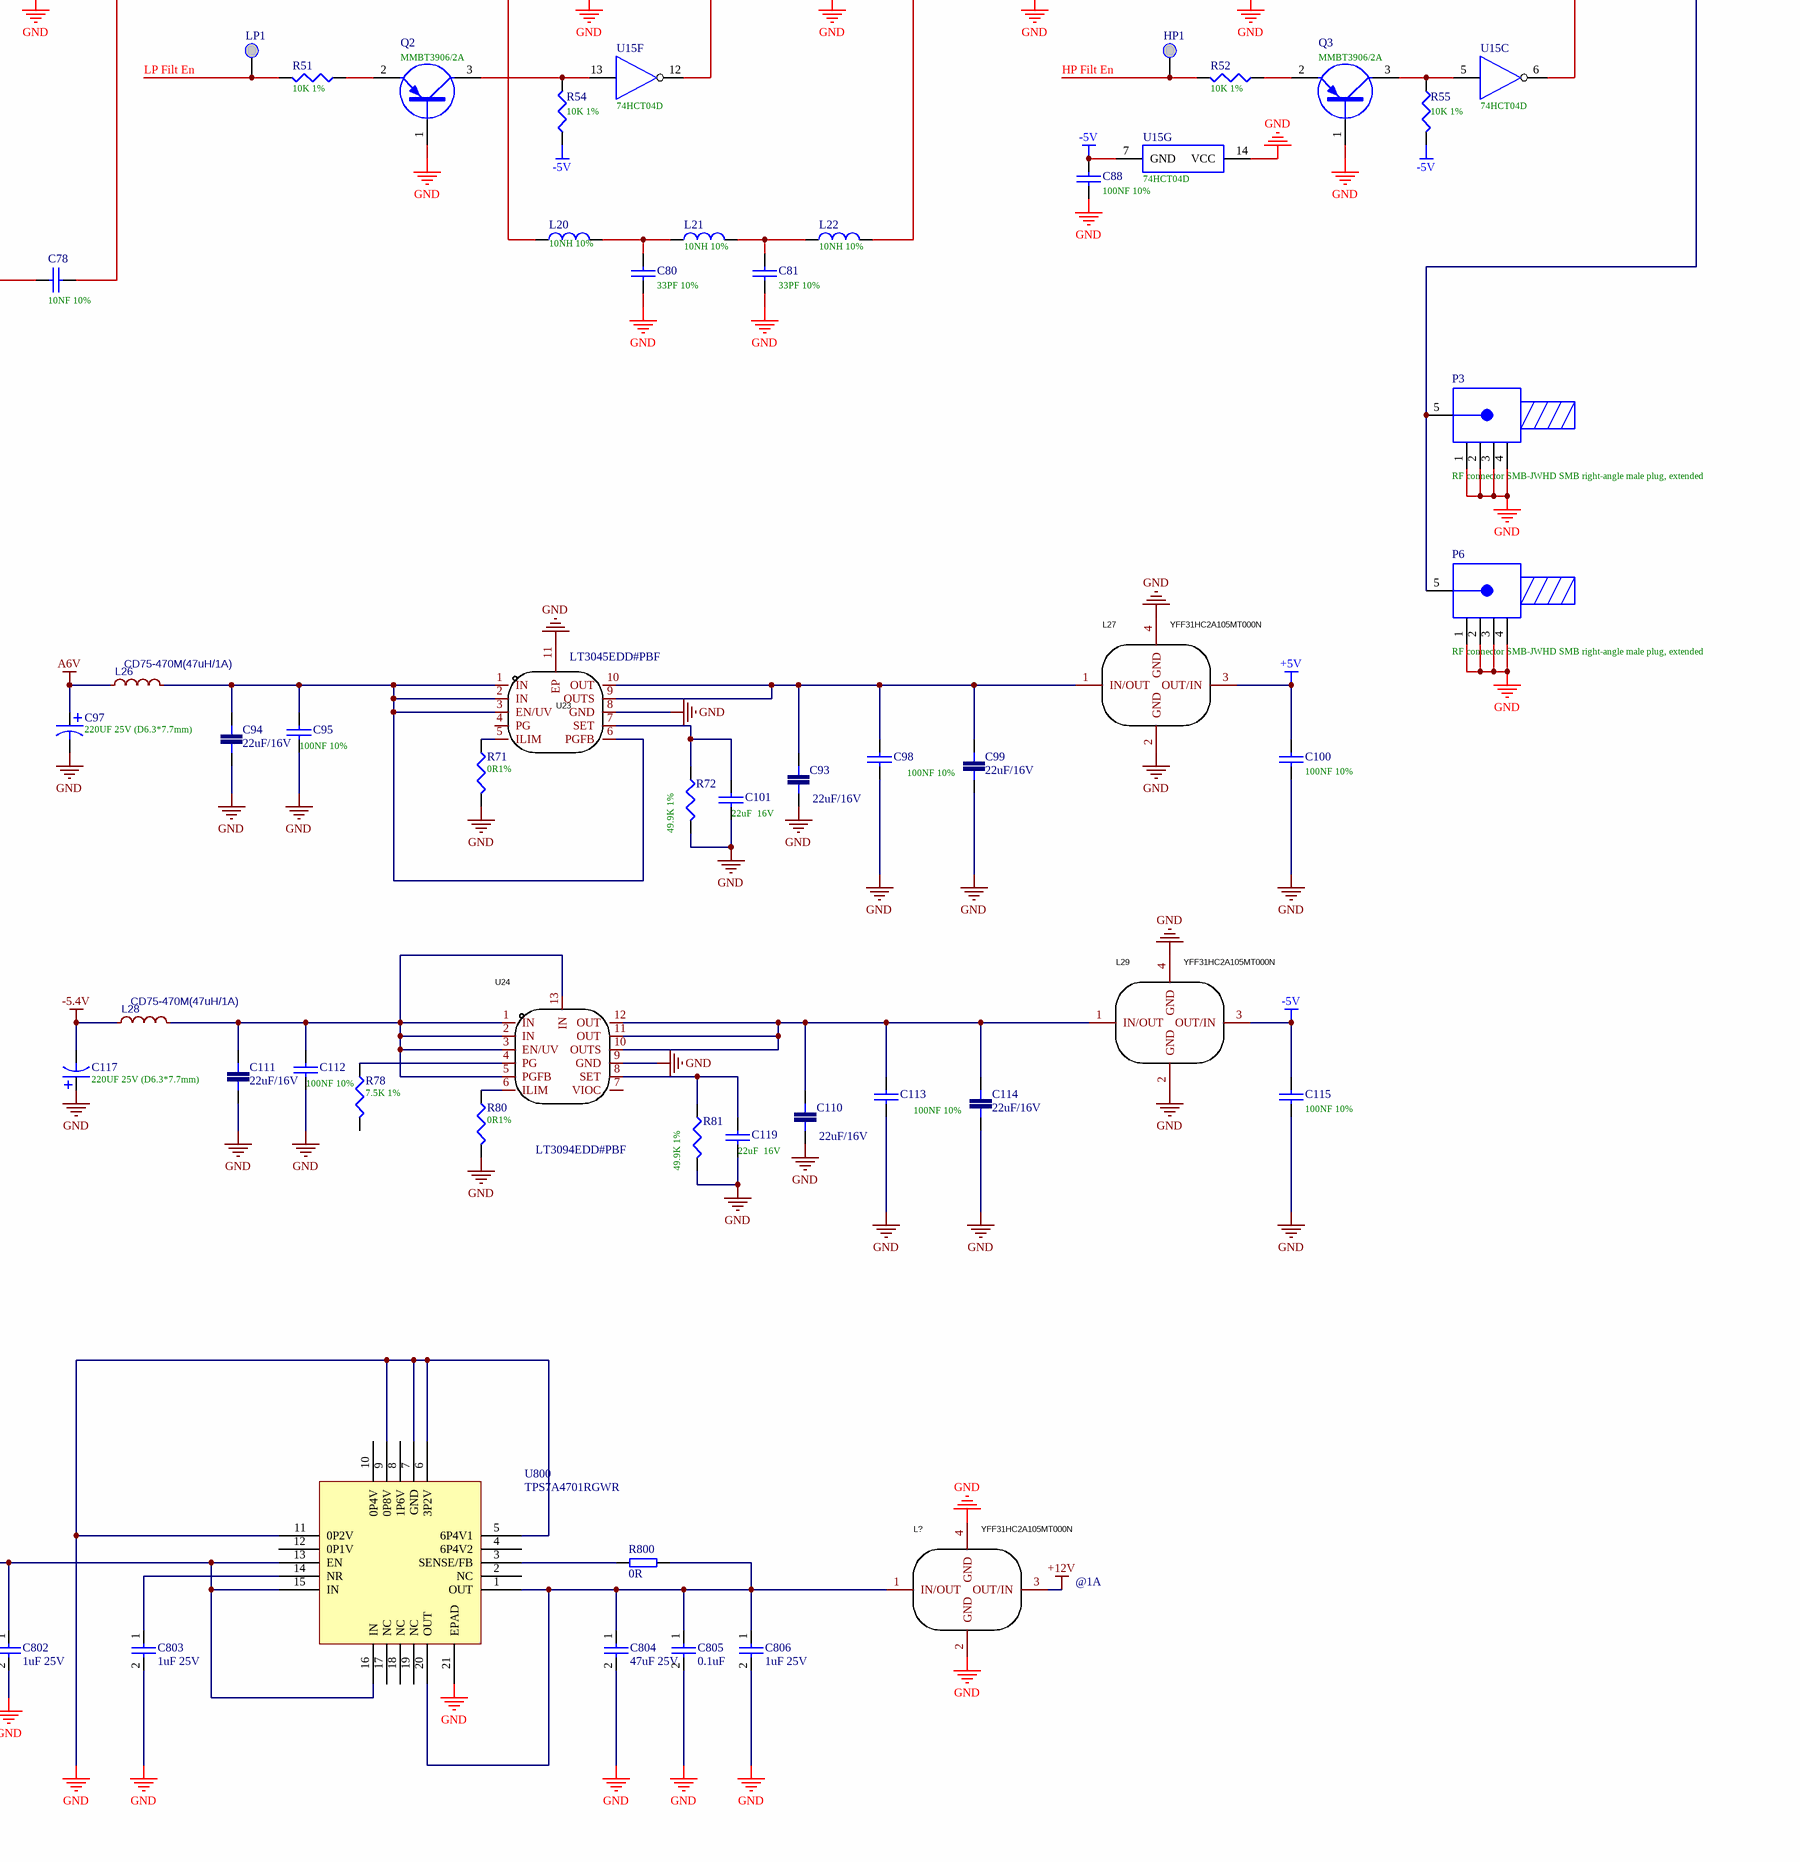
[diagram p0: PCBE109560.SchDoc, bottom right]
# Altium schematic sheet PCBE109560.SchDoc (part 2 of 2)

## Parts
1  (no value)  [DIP-1]
+1  (no value)  [DIP-1]
+2  (no value)  [DIP-1]
C4  20PF 10%  [0805C]
C5  330PF 10%  [1812C]
C6  22PF 10%  [1812C-2]
C7  22uF/16V  [0805]
C8  22uF/16V  [0805]
C9  100NF 10%  [0603]
C10  220UF 25V (D6.3*7.7mm)  [CAP-SMD_BD6.3-L6.6-W6.6-FD]
C11  100NF 10%  [0603]
C12  22uF/16V  [0805]
C13  100NF 10%  [0805R]
C14  22uF  16V  [0805]
C15  100NF 10%  [0805R]
C16  47PF 10%  [1812C-2]
C17  100PF 10%  [1812C-2]
C18  20PF 10%  [0805R]
C20  100NF 10%  [0805R]
C21  100NF 10%  [0805R]
C31  100NF 10%  [0805R]
C32  100NF 10%  [0805R]
C34  100NF 10%  [0805R]
C35  100NF 10%  [0805R]
C36  100NF 10%  [0805R]
C37  100NF 10%  [0805R]
C39  100NF 10%  [0805R]
C40  100NF 10%  [0805R]
C41  100NF 10%  [0805R]
C42  100NF 10%  [0805R]
C43  100NF 10%  [0805R]
C44  100NF 10%  [0805R]
C45  100NF 10%  [0805R]
C46  100NF 10%  [0805R]
C47  100NF 10%  [0805R]
C48  100NF 10%  [0805R]
C49  22uF 25V  [CAP-SMD_L6.0-W3.2-R-RD]
C50  100NF 10%  [0805R]
C51  100NF 10%  [0805R]
C52  100NF 10%  [0805R]
C53  3.3NF 10%  [0805R]
C54  100NF 10%  [0805R]
C55  330PF 10%  [0805R]
C56  330PF 10%  [0805R]
C57  100NF 10%  [0805R]
C58  33PF 10%  [0805R]
C59  33PF 10%  [0805R]
C60  100NF 10%  [0805R]
C61  100NF 10%  [0805R]
C62  100NF 10%  [0805R]
C63  100NF 10%  [0805R]
C64  100NF 10%  [0805R]
C65  33PF 10%  [0805R]
C66  33PF 10%  [0805R]
C67  100NF 10%  [0805R]
C68  39PF 10%  [0805R]
C69  100NF 10%  [0805R]
C70  25V 1UF Type A  [0805C-2]
C71  25V 1UF Type A  [0805C-2]
C72  100NF 10%  [0805R]
C73  25V 1UF Type A  [0805C-2]
C74  100NF 10%  [0805R]
C75  100NF 10%  [0805R]
C76  10NF 10%  [0805R]
C77  10NF 10%  [0805R]
C78  10NF 10%  [0805R]
C79  100NF 10%  [0603C]
C80  33PF 10%  [0805R]
C81  33PF 10%  [0805R]
C82  100NF 10%  [0805R]
C83  100NF 10%  [0805R]
C84  100NF 10%  [0805R]
C85  100NF 10%  [0805R]
C86  25V 1UF Type A  [0805C-2]
C87  3pF( ±0.1pF)  [0805R]
C88  100NF 10%  [0805R]
C89  100NF 10%  [0805R]
C90  100NF 10%  [0805R]
C93  22uF/16V  [0805]
C94  22uF/16V  [0805]
C95  100NF 10%  [0603]
C96  100NF 10%  [0805R]
C97  220UF 25V (D6.3*7.7mm)  [CAP-SMD_BD6.3-L6.6-W6.6-FD]
C98  100NF 10%  [0603]
C99  22uF/16V  [0805]
C100  100NF 10%  [0805R]
C101  22uF  16V  [0805]
C102  100NF 10%  [0805R]
C103  100NF 10%  [0805R]
C104  100NF 10%  [0805R]
C105  100NF 10%  [0805R]
C106  100NF 10%  [0805R]
C107  100NF 10%  [0805R]
C109  100NF 10%  [0805R]
C110  22uF/16V  [0805]
C111  22uF/16V  [0805]
C112  100NF 10%  [0603]
C113  100NF 10%  [0603]
C114  22uF/16V  [0805]
C115  100NF 10%  [0805R]
C116  100NF 10%  [0805R]
C117  220UF 25V (D6.3*7.7mm)  [CAP-SMD_BD6.3-L6.6-W6.6-FD]
C118  100NF 10%  [0805R]
C119  22uF  16V  [0805]
C122  100NF 10%  [0805R]
C123  100NF 10%  [0805R]
C124  100NF 10%  [0805R]
C125  100NF 10%  [0805R]
C128  100NF 10%  [0805R]
C129  100NF 10%  [0805R]
C130  100NF 10%  [0805R]
C800  47uF 25V  [1206]
C801  0.1uF  [0402]
C802  1uF 25V  [0402]
C803  1uF 25V  [0402]
C804  47uF 25V  [1206]
C805  0.1uF  [0402]
C806  1uF 25V  [0402]
Clk1  (no value)  [DIP-1]
D1  BAV99/A7  [SOT-23]
D2  GF1M-E3/67A/GM  [1808D]
D3  GF1M-E3/67A/GM  [1808D]
D4  GF1M-E3/67A/GM  [1808D]
D5  GF1M-E3/67A/GM  [1808D]
D8  BAV99/A7  [SOT-23-2]
D9  BAV99/A7  [SOT-23-2]
D10  BAV99/A7  [SOT-23-2]
D11  BAV99/A7  [SOT-23-2]
D12  BAV99/A7  [SOT-23-2]
Data1  (no value)  [DIP-1]
HP1  (no value)  [DIP-1]
J1  RF connector  [DIP-J-2]
J2  RF connector  [DIP-J-2]
L2  15UH 5%  [1005R]
L3  BLM21PG221SN1D(220Ω@100MHz)  [0805R]
L4  YFF31HC2A105MT000N  [FILTER-SMD_4P-L3.2-W1.6-L_YFF31HC]
L5  6.8UH 10%  [0805R]
L8  YFF31HC2A105MT000N  [FILTER-SMD_4P-L3.2-W1.6-L_YFF31HC]
L9  BLM21PG221SN1D(220Ω@100MHz  [0805R]
L10  10NH 10%  [0805R]
L11  10NH 10%  [0805R]
L12  10NH 10%  [0805R]
L13  YFF31HC2A105MT000N  [FILTER-SMD_4P-L3.2-W1.6-L_YFF31HC]
L14  BLM21PG221SN1D(220Ω@100MHz  [0805R]
L15  4.7UH 5%  [1005L]
L16  1UH 5%  [0805R]
L17  BLM21PG221SN1D(220Ω@100MHz)  [0805R]
L18  BLM21PG221SN1D(220Ω@100MHz  [0805R]
L19  BLM21PG221SN1D(220Ω@100MHz  [0805R]
L20  10NH 10%  [0805R]
L21  10NH 10%  [0805R]
L22  10NH 10%  [0805R]
L23  YFF31HC2A105MT000N  [FILTER-SMD_4P-L3.2-W1.6-L_YFF31HC]
L24  YFF31HC2A105MT000N  [FILTER-SMD_4P-L3.2-W1.6-L_YFF31HC]
L25  BLM21PG221SN1D(220Ω@100MHz  [0805R]
L26  CD75-470M(47uH/1A)  [IND-SMD_L7.8-W7.0-A]
L27  YFF31HC2A105MT000N  [FILTER-SMD_4P-L3.2-W1.6-L_YFF31HC]
L28  CD75-470M(47uH/1A)  [IND-SMD_L7.8-W7.0-A]
L29  YFF31HC2A105MT000N  [FILTER-SMD_4P-L3.2-W1.6-L_YFF31HC]
L31  BLM21PG221SN1D(220Ω@100MHz  [0805R]
L32  BLM21PG221SN1D(220Ω@100MHz  [0805R]
L808  NFM15PC104R1A3D  [FILTER-SMD_0402-3P-L1.0-W0.5-T]
L809  NFM15PC104R1A3D  [FILTER-SMD_0402-3P-L1.0-W0.5-T]
L810  NFM15PC104R1A3D  [FILTER-SMD_0402-3P-L1.0-W0.5-T]
L811  NFM15PC104R1A3D  [FILTER-SMD_0402-3P-L1.0-W0.5-T]
L812  NFM15PC104R1A3D  [FILTER-SMD_0402-3P-L1.0-W0.5-T]
L813  NFM15PC104R1A3D  [FILTER-SMD_0402-3P-L1.0-W0.5-T]
L?  YFF31HC2A105MT000N  [FILTER-SMD_4P-L3.2-W1.6-L_YFF31HC]
LP1  (no value)  [DIP-1]
P1  Header 20X2  [N0.8mm/40Pin-Plug]
P2  Header 4X2  [N0.8mm/8Pin-SOCKET]
P3  RF connector SMB-JWHD SMB right-angle male plug, extended  [DIP-P-2]
P4  Header 20X2  [N0.8mm/40Pin-Plug]
P5  Header 20X2  [N0.8mm/40Pin-Plug]
P6  RF connector SMB-JWHD SMB right-angle male plug, extended  [DIP-P-2]
Q1  MJD31C  [SOT-252-2]
Q2  MMBT3906/2A  [SOT-23]
Q3  MMBT3906/2A  [SOT-23]
Q4  MMBT3906/2A  [SOT-23]
R6  2K 5%  [0603R]
R7  NC  [AXIAL-0.51]
R8  3.9K 5% 1/2W  [AXIAL-0.51]
R9  3.9K 5% 1/2W  [AXIAL-0.51]
R10  3.9K 5% 1/2W  [AXIAL-0.51]
R11  3.9K 5% 1/2W  [AXIAL-0.51]
R13  0R1%  [0603]
R14  49.9K 1%  [0603]
R15  4.99K 1%  [0805R]
R16  2K 1%  [0805R]
R17  49.9R 1% 1/4W  [AXIAL-0.4]
R20  100R 1% 1/4W  [AXIAL-0.4]
R23  100R 1% 1/4W  [AXIAL-0.4]
R27  4.87K 1%  [0805R]
R28  4.87K 1%  [0805R]
R29  4.87K 1%  [0805R]
R30  4.87K 1%  [0805R]
R31  4.87K 1%  [0805R]
R32  10K 1%  [0805R]
R33  100K 1%  [0805R]
R34  100K 1%  [0805R]
R35  49.9R 1%  [0805R]
R36  49.9R 1%  [0805R]
R37  49.9R 1%  [0805R]
R38  49.9R 1%  [0805R]
R39  49.9R 1%  [0805R]
R40  49.9R 1% 1/4W  [R-SMD_L3.5-W1.5]
R41  10K 1%  [0805R]
R42  4.87K 1%  [0805R]
R43  4.87K 1%  [0805R]
R44  4.87K 1%  [0805R]
R45  4.87K 1%  [0805R]
R46  169R 1%  [0805R]
R47  169R 1%  [0805R]
R48  169R 1%  [0805R]
R49  49.9R 1%  [0805R]
R50  49.9R 1%  [0805R]
R51  10K 1%  [0805R]
R52  10K 1%  [0805R]
R53  10K 1%  [0805R]
R54  10K 1%  [0805R]
R55  10K 1%  [0805R]
R56  10K 1%  [0805R]
R57  10K 1%  [0805R]
R58  49.9R 1%  [0805R]
R59  4.99K 1%  [0805R]
R60  49.9R 1%  [R-SMD_L3.5-W1.5]
R61  30R 1%  [R-SMD_L3.5-W1.5]
R62  169R 1%  [0805R]
R63  169R 1%  [0805R]
R64  169R 1%  [0805R]
R65  49.9R 1%  [0805R]
R66  49.9R 1%  [0805R]
R67  49.9R 1%  [0805R]
R68  49.9R 1%  [0805R]
R69  120R 1%  [R-SMD_L3.5-W1.5]
R70  169R 1%  [0805R]
R71  0R1%  [0603]
R72  49.9K 1%  [0603]
R73  169R 1%  [0805R]
R74  NC  [0805R]
R75  169R 1%  [0805R]
R77  169R 1%  [0805R]
R78  7.5K 1%  [0603]
R80  0R1%  [0603]
R81  49.9K 1%  [0603]
R82  100K 1%  [0805R]
R83  10K 1%  [0805R]
R84  169R 1%  [0805R]
R800  0R  [0402]
RE1  AGQ210A4HZ  [RELAY-SMD_PANASONIC_AGQ2X0AXX]
RE2  AGQ210A4HZ  [RELAY-SMD_PANASONIC_AGQ2X0AXX]
RE3  AGQ210A4HZ  [RELAY-SMD_PANASONIC_AGQ2X0AXX]
RE4  AGQ210A4HZ  [RELAY-SMD_PANASONIC_AGQ2X0AXX]
RE5  AGQ210A4HZ  [RELAY-SMD_PANASONIC_AGQ2X0AXX]
Strobe1  (no value)  [DIP-1]
U4  LT3045EDD#PBF  [DFN-10_L3.0-W3.0-P0.50-BL-EP]
U6  74HCT123D  [SOIC-16_L9.9-W3.9-P1.27-LS6.0-BL]
U8  MAX504CSD+T  [SO-14]
U9  SW-239  [SO-8]
U11  SW-239  [SO-8]
U12  SW-239  [SO-8]
U13  SW-239  [SO-8]
U14  SW-239  [SO-8]
U15  74HCT04D  [SO-14]  (parts A,B,C,D,E,F,G of 7)
U16  AT-250(MAAV-007941)  [SO-8]
U17  MAR-3SM/A03  [LCC4]
U18  MAR-6SM/A06  [LCC4]
U19  MAR-6SM/A06  [LCC4]
U20  MAR-3SM/A03  [LCC4]
U21  MAX4106ESA+T  [SO-8]
U22  MIC4420CM  [SO-8]
U23  LT3045EDD#PBF  [DFN-10_L3.0-W3.0-P0.50-BL-EP]
U24  LT3094EDD#PBF  [WDFN-12_L3.0-W3.0-P0.45-BL-EP]
U25  AT65-0263  [SO-16]
U100  SW-239  [SO-8]
U800  TPS7A4701RGWR  [QFN-20]

## Nets
+5V: C100.1 L27.3(OUT/IN) L808.3(OUTPUT) L811.3(OUTPUT) L812.3(OUTPUT) U8.3(~{CLR})
+12.5V: +2.1 C106.1 C800.1 C801.1 C802.1 P5.31 P5.32 P5.33 P5.34 P5.35 P5.36 P5.37 P5.38 P5.39 P5.40 U800.13(EN) U800.15(IN) U800.16(IN)
+12V: C122.1 C123.1 C124.2 C125.2 L8.1(IN/OUT) L13.1(IN/OUT) L?.3(OUT/IN) U22.1(VS) U22.8(VS)
-5.4V: +1.1 C107.1 C117.2 L28.2 P5.1 P5.2 P5.3 P5.4 P5.5 P5.6 P5.7 P5.8 P5.9 P5.10
-5V: C88.2 C115.2 L29.3(OUT/IN) L809.1(INPUT) L810.3(OUTPUT) L813.3(OUTPUT) R54.1 R55.2 R57.1 U15.7(GND)
A6V: 1.1 C10.1 C97.1 C103.2 L3.1 L26.2 P5.17 P5.18 P5.19 P5.20 P5.21 P5.22 P5.23 P5.24
GND: C5.1 C6.2 C7.1 C8.1 C9.2 C10.2 C11.2 C12.1 C13.2 C14.2 C15.1 C18.2 C20.1 C21.1 C31.1 C32.1 C34.1 C35.1 C36.2 C37.2 C39.2 C40.2 C42.2 C43.1 C44.2 C45.2 C46.2 C47.1 C48.1 C49.2 C50.2 C57.2 C60.2 C61.1 C62.1 C63.1 C64.1 C65.2 C66.1 C70.1 C71.1 C72.2 C73.1 C74.1 C75.1 C80.1 C81.1 C83.2 C84.2 C85.1 C86.2 C88.1 C89.2 C90.2 C93.1 C94.1 C95.2 C96.2 C97.2 C98.2 C99.1 C100.2 C101.2 C102.2 C103.1 C104.2 C105.1 C106.2 C107.2 C109.2 C110.1 C111.1 C112.2 C113.2 C114.1 C115.1 C117.1 C118.2 C119.2 C122.2 C123.2 C124.1 C125.1 C128.1 C129.1 C130.2 C800.2 C801.2 C802.2 C803.2 C804.2 C805.2 C806.2 D1.3 D2.2(K) D11.2 D12.1 J1.1 J1.2 J1.3 J1.4 J2.1 J2.2 J2.3 J2.4 L2.2 L4.2(GND) L4.4(GND) L8.2(GND) L8.4(GND) L13.2(GND) L13.4(GND) L15.2 L16.1 L23.2(GND) L23.4(GND) L24.2(GND) L24.4(GND) L27.2(GND) L27.4(GND) L29.2(GND) L29.4(GND) L808.2(GND) L809.2(GND) L810.2(GND) L811.2(GND) L812.2(GND) L813.2(GND) L?.2(GND) L?.4(GND) P1.5 P1.6 P1.11 P1.12 P1.17 P1.18 P1.20 P1.23 P1.24 P1.29 P1.30 P1.35 P1.36 P2.1 P2.3 P2.5 P2.7 P3.1 P3.2 P3.3 P3.4 P4.5 P4.6 P4.11 P4.12 P4.17 P4.18 P4.23 P4.24 P4.29 P4.30 P4.35 P4.36 P5.11 P5.12 P5.13 P5.14 P5.15 P5.16 P5.25 P5.26 P5.27 P5.28 P5.29 P5.30 P6.1 P6.2 P6.3 P6.4 Q1.2(E) Q2.1(B) Q3.1(B) Q4.1(B) R13.2 R14.2 R20.2 R32.2 R53.1 R59.1 R61.1 R71.2 R72.2 R74.1 R80.2 R81.2 R82.1 R83.1 RE1.3 RE3.6 RE4.2 U4.8(GND) U4.11(EP) U6.6(2CEXT) U6.8(GND) U6.10(2B) U6.14(1CEXT) U8.7(DGND) U8.8(AGND) U9.2(GND) U9.7(GND) U9.8(GND) U11.2(GND) U11.7(GND) U11.8(GND) U12.2(GND) U12.7(GND) U12.8(GND) U13.2(GND) U13.7(GND) U13.8(GND) U14.2(GND) U14.7(GND) U14.8(GND) U15.14(VCC) U16.2(GND) U16.3(GND) U16.5(GND) U16.6(GND) U16.7(GND) U17.2(GND) U17.4(GND) U18.2(GND) U18.4(GND) U19.2(GND) U19.4(GND) U20.2(GND) U20.4(GND) U22.4(GND) U22.5(GND) U23.8(GND) U23.11(EP) U24.9(GND) U25.2(GND) U25.3(GND) U25.4(GND) U25.5(GND) U25.6(GND) U25.7(GND) U25.16(GND) U100.2(GND) U100.7(GND) U100.8(GND) U800.5(6P4V1) U800.6(3P2V) U800.7(GND) U800.9(0P8V) U800.11(0P2V) U800.21(EPAD)
VCC: C13.1 C15.2 L4.3(OUT/IN) R15.1 R16.2 U6.2(1B) U6.3(1~{R}D) U6.16(VCC)
AK2: C21.2 P1.33 RE1.1
AK3: C20.2 P1.38 RE1.8
AK4: C37.1 P1.37 RE2.1
AK5: C36.1 P1.40 RE2.8
AK6: C31.2 P1.34 RE3.8
AK7: C32.2 P1.32 RE3.1
AK8: C34.2 C40.1 P1.28 RE4.8 RE5.8
AK9: C35.2 C39.1 P1.26 RE4.1 RE5.1
Attn1: P4.34 R70.2
Attn2: P4.32 R73.2
Attn4: P4.28 R75.2
Attn8: P4.26 R77.2
Attn16: P4.22 R84.2
DAC Clk: Clk1.1 P4.14 U8.4(SCLK)
DAC Data: Data1.1 P4.16 U8.2(DIN)
DAC Strobe: P4.10 Strobe1.1 U8.5(~{CS})
DATA_T: P1.39 R15.2 U6.1(1~{A})
HP Filt En: HP1.1 P4.4 R52.2
HT: L5.1 P2.2 P2.4 P2.6 P2.8
IN2: P4.8 R56.1 U22.2(IN)
LP Filt En: LP1.1 P4.2 R51.2
NetC4_1: C4.1 D1.2 L2.1 Q1.1(B) R6.1
NetC4_2: C4.2 R6.2 U6.13(1Q)
NetC5_2: C5.2 L5.2 R7.2
NetC6_1: C6.1 C16.2 C17.2 Q1.3(C) R11.1
NetC7_2: C7.2 C11.1 C12.2 L4.1(IN/OUT) U4.9(OUTS) U4.10(OUT)
NetC8_2: C8.2 C9.1 L3.2 U4.1(IN) U4.2(IN) U4.3(EN/UV) U4.6(PGFB)
NetC14_1: C14.1 R14.1 U4.7(SET)
NetC16_1: C16.1 D5.1(A) D8.2 D9.2 RE2.6
NetC17_1: C17.1 RE2.7
NetC18_1: C18.1 R16.1 U6.15(1REXT/CEXT)
NetC41_1: C41.1 U14.1(RFCOM)
NetC41_2: C41.2 P3.5 P6.5 R32.1
NetC42_1: C42.1 R27.1 U9.5(B)
NetC43_2: C43.2 R28.2 U100.4(A)
NetC44_1: C44.1 R29.1 U11.4(A)
NetC45_1: C45.1 R30.1 U12.5(B)
NetC46_1: C46.1 R31.1 U13.5(B) U14.4(A)
NetC47_2: C47.2 R35.1 U16.4(A)
NetC48_2: C48.2 L8.3(OUT/IN) R36.1
NetC49_1: C49.1 C50.1 U8.1(BIPOFF) U8.9(REFIN) U8.10(REFOUT)
NetC51_1: C51.1 U17.1(RF_IN)
NetC51_2: C51.2 U16.8(RF2)
NetC52_1: C52.1 L10.2
NetC52_2: C52.2 L9.1 U17.3(RF_OUT)
NetC53_1: C53.1 C54.1 L15.1
NetC53_2: C53.2 U12.1(RFCOM)
NetC54_2: C54.2 U13.1(RFCOM)
NetC55_1: C55.1 U13.3(RF1)
NetC55_2: C55.2 C56.1 L16.2
NetC56_2: C56.2 U14.6(RF2)
NetC57_1: C57.1 R41.1 U13.4(A) U14.5(B)
NetC58_1: C58.1 C65.1
NetC58_2: C58.2 L10.1 L11.1
NetC59_1: C59.1 L11.2 L12.1
NetC59_2: C59.2 C66.2
NetC60_1: C60.1 R42.1 U9.4(A)
NetC61_2: C61.2 R43.2 U100.5(B)
NetC62_2: C62.2 R44.1 U11.5(B)
NetC63_2: C63.2 R45.1 U12.4(A)
NetC64_2: C64.2 L13.3(OUT/IN) R46.2
NetC67_1: C67.1 U18.1(RF_IN)
NetC67_2: C67.2 U25.1(RF)
NetC68_1: C68.1 C69.2 R49.2 R50.2
NetC68_2: C68.2 L14.2 R49.1 R50.1 U18.3(RF_OUT)
NetC69_1: C69.1 R53.2 U16.1(RF1)
NetC70_2: C70.2 C74.2 L18.1 L19.2
NetC71_2: C71.2 C75.2 L19.1 U21.4(VEE)
NetC72_1: C72.1 C73.2 L17.2 L18.2
NetC76_1: C76.1 U9.3(RF1)
NetC76_2: C76.2 U19.1(RF_IN)
NetC77_1: C77.1 R64.1 U19.3(RF_OUT)
NetC77_2: C77.2 U20.1(RF_IN)
NetC78_1: C78.1 R68.2 U20.3(RF_OUT)
NetC78_2: C78.2 U100.6(RF2)
NetC79_1: C79.1 D10.3 R40.2
NetC79_2: C79.2 R58.2 R59.2
NetC80_2: C80.2 L20.2 L21.2
NetC81_2: C81.2 L21.1 L22.1
NetC82_1: C82.1 R60.2
NetC82_2: C82.2 C116.1 R74.2 R82.2
NetC83_1: C83.1 C86.1 L25.2 U21.7(VCC)
NetC84_1: C84.1 L23.3(OUT/IN) R62.2
NetC85_2: C85.2 L24.3(OUT/IN) R65.1
NetC87_1: C87.1 R60.1 R69.1 U21.6(OUT)
NetC87_2: C87.2 R61.2 R69.2 U21.2(IN-)
NetC89_1: C89.1 L813.1(INPUT) U8.11(VSS)
NetC90_1: C90.1 L32.2 L811.1(INPUT)
NetC93_2: C93.2 C98.1 C99.2 L27.1(IN/OUT) U23.9(OUTS) U23.10(OUT)
NetC94_2: C94.2 C95.1 L26.1 U23.1(IN) U23.2(IN) U23.3(EN/UV) U23.6(PGFB)
NetC96_1: C96.1 R70.1 U25.15(C1)
NetC101_1: C101.1 R72.1 U23.7(SET)
NetC102_1: C102.1 R73.1 U25.14(C2)
NetC104_1: C104.1 L812.1(INPUT) U8.13(VDD)
NetC105_2: C105.2 L31.1 L810.1(INPUT)
NetC109_1: C109.1 R75.1 U25.13(C4)
NetC110_2: C110.2 C113.1 C114.2 L29.1(IN/OUT) U24.10(OUTS) U24.11(OUT) U24.12(OUT)
NetC111_2: C111.2 C112.1 L28.1 U24.1(IN) U24.2(IN) U24.3(EN/UV) U24.5(PGFB) U24.13(IN)
NetC116_2: C116.2 R83.2 U25.8(RF)
NetC118_1: C118.1 R77.1 U25.12(C8)
NetC119_1: C119.1 R81.1 U24.8(SET)
NetC128_2: C128.2 L31.2 U25.11(VEE)
NetC129_2: C129.2 L32.1 U25.10(VCC)
NetC130_1: C130.1 R84.1 U25.9(C16)
NetC803_1: C803.1 U800.14(NR)
NetC804_1: C804.1 C805.1 C806.1 L?.1(IN/OUT) R800.1 U800.1(OUT) U800.20(OUT)
NetD2_1: D2.1(A) D3.2(K)
NetD3_1: D3.1(A) D4.2(K)
NetD4_1: D4.1(A) D5.2(K)
NetD8_1: D8.1 D9.1 J1.5 R17.1 R20.1 R23.1 RE4.4
NetD10_1: D10.1 D12.2
NetD10_2: D10.2 D11.1
NetJ2_5: J2.5 RE5.4
NetL9_2: L9.2 R39.2
NetL12_2: L12.2 U9.1(RFCOM)
NetL14_1: L14.1 R48.2
NetL17_1: L17.1 L809.3(OUTPUT)
NetL20_1: L20.1 U11.6(RF2)
NetL22_2: L22.2 U12.3(RF1)
NetL23_1: L23.1(IN/OUT) L24.1(IN/OUT) U22.6(OUT) U22.7(OUT)
NetL25_1: L25.1 L808.1(INPUT)
NetQ2_2: Q2.2(E) R51.1
NetQ2_3: Q2.3(C) R54.2 U15.13(6A)
NetQ3_2: Q3.2(E) R52.1
NetQ3_3: Q3.3(C) R55.1 U15.5(3A)
NetQ4_2: Q4.2(E) R56.2
NetQ4_3: Q4.3(C) R57.2 U15.1(1A)
NetR7_1: R7.1 R8.1
NetR8_2: R8.2 R9.2
NetR9_1: R9.1 R10.1
NetR10_2: R10.2 R11.2
NetR13_1: R13.1 U4.5(ILIM)
NetR17_2: R17.2 RE1.2
NetR23_2: R23.2 RE3.7
NetR27_2: R27.2 R28.1 U15.4(2Y)
NetR29_2: R29.2 R30.2 U15.10(5Y)
NetR31_2: R31.2 U15.8(4Y)
NetR33_1: R33.1 R34.1 U8.14(RFB)
NetR33_2: R33.2 R34.2 R35.2 U8.12(VOUT)
NetR36_2: R36.2 R37.1
NetR37_2: R37.2 R38.2
NetR38_1: R38.1 R39.1
NetR40_1: R40.1 RE5.3
NetR41_2: R41.2 U15.6(3Y) U15.9(4A)
NetR42_2: R42.2 R43.1 U15.2(1Y) U15.3(2A)
NetR44_2: R44.2 R45.2 U15.11(5A) U15.12(6Y)
NetR46_1: R46.1 R47.2
NetR47_1: R47.1 R48.1
NetR58_1: R58.1 U21.3(IN+)
NetR62_1: R62.1 R63.1
NetR63_2: R63.2 R64.2
NetR65_2: R65.2 R66.2
NetR66_1: R66.1 R67.1
NetR67_2: R67.2 R68.1
NetR71_1: R71.1 U23.5(ILIM)
NetR78_1: R78.1 U24.4(PG)
NetR80_1: R80.1 U24.6(ILIM)
NetR800_2: R800.2 U800.3(SENSE/FB)
NetRE4_3: RE4.3 RE5.2
NetU9_6: U9.6(RF2) U100.3(RF1)
NetU11_1: U11.1(RFCOM) U100.1(RFCOM)
NetU11_3: U11.3(RF1) U12.6(RF2)
NetU13_6: U13.6(RF2) U14.3(RF1)

Not connected (* = marked no-connect by the designer): D1 1*; D8 3; D9 3; D11 3; D12 3; P1 1 2 3 4 7 8 9 10 13 14 15 16 19 21 22 25 27 31; P4 1 3 7 9 13 15 19 20 21 25 27 31 33 37 38 39 40; R78 2; RE1 4 5 6 7; RE2 2 3 4 5; RE3 2 3 4 5; RE4 5 6 7; RE5 5 6 7; U4 4(PG); U6 4(1~{Q}) 5(2Q) 7(2REXT/CEXT) 9(2~{A}) 11(2~{R}D) 12(2~{Q}); U8 6(DOUT); U22 3(NC); U23 4(PG); U24 7(VIOC); U800 2(NC) 4(6P4V2) 8(1P6V) 10(0P4V) 12(0P1V) 17(NC) 18(NC) 19(NC)

## Notes on the sheet
- (near P1) Transmit interface
- 500V high-voltage interface
- Receive interface
- @1A

## Library data of the parts
1 +1 +2 Clk1 Data1 HP1 LP1 Strobe1 = TP
C4-C6 C9 C11 C13-C18 C20 C21 C31 C32 C34-C37 C39-C48 C50-C69 C72-C85 C87-C90 C95 C96 C98 C100-C107 C109 C112 C113 C115 C116 C118 C119 C122-C125 C128-C130 C800-C806 = CAP: Capacitor
C7 C8 C12 C93 C94 C99 C110 C111 C114 = C1206
C10 C97 C117 = CAPACITOR_1: Capacitor
C49 = TAJC226K025RNJ: Manufacturer: Kyocera AVX; Add into BOM: yes; Tolerance: ±10%; Equivalent Series Resistance(ESR): 1.4Ω@100kHz; Symbol: TAJC226K025RNJ; Device: TAJC226K025RNJ; LCSC Part Name: 22uF ±10% 25V; Supplier Part: C7214; Manufacturer Part: TAJC226K025RNJ; Supplier Footprint: CASE-C-6032; JLCPCB Part Class: Extended Part; Datasheet: https://atta.szlcsc.com/upload/public/pdf/source/20160107/1457707750344.pdf; Supplier: LCSC; Convert to PCB: yes; Value: 22uF; Rated Voltage: 25V; Operating Temperature: -55℃~+125℃
C70 C71 C86 = CAPACITOR POL: Capacitor
D1 D8-D12 = BAV99
D2-D5 = DIODE
J1 J2 = SMA-KWE: BOM_Supplier: *; BOM_Supplier Part: *; BOM_Manufacturer: *; BOM_Manufacturer Part: *; BOM_JLCPCB Part Class: *; spicePre: *; spiceSymbolName: *; Contributor: *
L2 L3 L5 L9-L12 L14-L22 L25 L31 L32 = INDUCTOR
L4 L8 L13 L23 L24 L27 L29 L? = YFF31HC2A105MT000N: Manufacturer: TDK; Add into BOM: yes; Nominal Capacitance: 1uF; CapacitanceTolerance: ±20%; DC Rated Voltage: 100V; Rated Current: 6A; DC Resistance: 5mΩ; Name: YFF31HC2A105MT000N; Symbol: YFF31HC2A105MT000N; Device: YFF31HC2A105MT000N; LCSC Part Name: 1uF(105) ±20% 100V; Supplier Part: C113216; Manufacturer Part: YFF31HC2A105MT000N; Supplier Footprint: SMD-4P,1.6x3.2mm; JLCPCB Part Class: Extended Part; Datasheet: https://atta.szlcsc.com/upload/public/pdf/source/20180326/C113216_F6F81E50B9805DA3D7C436129903DEBD.pdf; Supplier: LCSC; Convert to PCB: yes; Operating Temperature: -55℃~+125℃
L26 L28 = 4.7uH/5a: BOM_Manufacturer: COILMX; BOM_Manufacturer Part: MS0630-4R7M; nameAlias: Inductance; Contributor: LCSC; BOM_Supplier: LCSC; BOM_Supplier Part: C380177; spicePre: L; spiceSymbolName: MS0630-4R7M
L808-L813 = NFM15PC104R1A3D: Manufacturer: muRata(村田); Add into BOM: yes; Nominal Capacitance: 100nF; CapacitanceTolerance: ±20%; DC Rated Voltage: 10V; Rated Current: 2A; DC Resistance: 30mΩ; Symbol: NFM15PC104R1A3D; Device: NFM15PC104R1A3D; LCSC Part Name: 0.1uF ±20% 10V; Supplier Part: C2650905; Manufacturer Part: NFM15PC104R1A3D; Supplier Footprint: 0402; JLCPCB Part Class: Extended Part; Datasheet: https://atta.szlcsc.com/upload/public/pdf/source/20210611/05FD8D968916F804F398094FB2B4AAFE.pdf; Supplier: LCSC; Convert to PCB: yes; Operating Temperature: -55℃~+105℃; Comment_1: NFM15PC104R1A3D
P1 P4 P5 = Header 20X2: Header, 20-Pin, Dual row; LatestRevisionDate: 17-Jul-2002; LatestRevisionNote: Re-released for DXP Platform.; Publisher: Altium Limited
P2 = Header 4X2: Header, 4-Pin, Dual row; LatestRevisionDate: 17-Jul-2002; LatestRevisionNote: Re-released for DXP Platform.; Publisher: Altium Limited
P3 P6 = JA1
Q1 = NPN: NPN Transistor
Q2-Q4 = PNP: PNP Transistor
R6-R11 R13-R17 R20 R23 R27-R75 R77 R78 R80-R84 = RES1
R800 = RES
RE1-RE5 = AGQ210A4HZ: Manufacturer: PANASONIC(松下); Add into BOM: yes; Coil Voltage: 4.5V; Contact Form: Two changeover sets: 2C (DPDT changeover); Maximum Switching Voltage: 125V@AC; 110V@DC; Coil Type: Single coil; Maximum Switching Current: 2A; Operate Time: 4ms; Symbol: AGQ210A4HZ; Device: AGQ210A4HZ; LCSC Part Name: AGQ210A4HZ; Supplier Part: C2153577; Manufacturer Part: AGQ210A4HZ; Supplier Footprint: SMD,7.2x10.6mm; JLCPCB Part Class: Extended Part; Datasheet: https://atta.szlcsc.com/upload/public/pdf/source/20210727/C2858037_82AE1FE69E1888D41D6E9B5D42950540.pdf; Supplier: LCSC; Convert to PCB: yes; Pin Number: -; Contact Rating: -; Contact Material: AgPd + gold plating; Coil Rated Power: -; Coil Resistance: -; Release Time: 4ms; Contact Resistance: -; Operating Temperature: -40℃~+85℃; Comment_1: AGQ210A4HZ
U4 U23 = LT3045EDD#PBF: Symbol: LT3045EDD#PBF_C666574; Add into BOM: yes; Maximum Input Voltage: 20V; Output Voltage: 0V~15V; MAX Output Current: 500mA; Dropout Voltage: 450mV@(500mA); standby current: 20uA; Number of Outputs: 1; Device: LT3045EDD#PBF; LCSC Part Name: LT3045EDD#PBF; Supplier Part: C666574; Manufacturer Part: LT3045EDD#PBF; Supplier Footprint: DFN-10-EP(3x3); JLCPCB Part Class: Extended Part; Datasheet: https://atta.szlcsc.com/upload/public/pdf/source/20200416/C514420_E440C492D6C74EAE6AB301243586F696.pdf; Supplier: LCSC; Convert to PCB: yes
U15 = 74HC04
U16 = AT-250
U17 U20 = MAR-3SM
U18 U19 = MAR-6SM
U21 = MAX4107ESA: Manufacturer: *; Manufacturer Part: *; Supplier Part: *; Supplier: *; link: *; spicePre: *; spiceSymbolName: *; Package Display: *; Contributor: *
U24 = LT3094EDD#PBF: Add into BOM: yes; Symbol: LT3094EDD#PBF; Device: LT3094EDD#PBF; LCSC Part Name: LT3094EDD#PBF; Supplier Part: C670492; Manufacturer Part: LT3094EDD#PBF; Supplier Footprint: WDFN-12-EP(3x3); JLCPCB Part Class: Extended Part; Datasheet: https://atta.szlcsc.com/upload/public/pdf/source/20200318/C498217_A5485280C797CF3891C55BEBE66C21D4.pdf; Supplier: LCSC; Convert to PCB: yes; Output Type: -
U800 = TPS7A4701RGWR(QFN20): Name: *; Symbol: *; Device: *; LCSC Part Name: *; Supplier Part: *; Manufacturer: *; Manufacturer Part: *; Supplier Footprint: *; JLCPCB Part Class: *; Datasheet: *; Supplier: *; Add into BOM: *; Convert to PCB: *; Output Type: *; Output Polarity: *; Number of Outputs: *